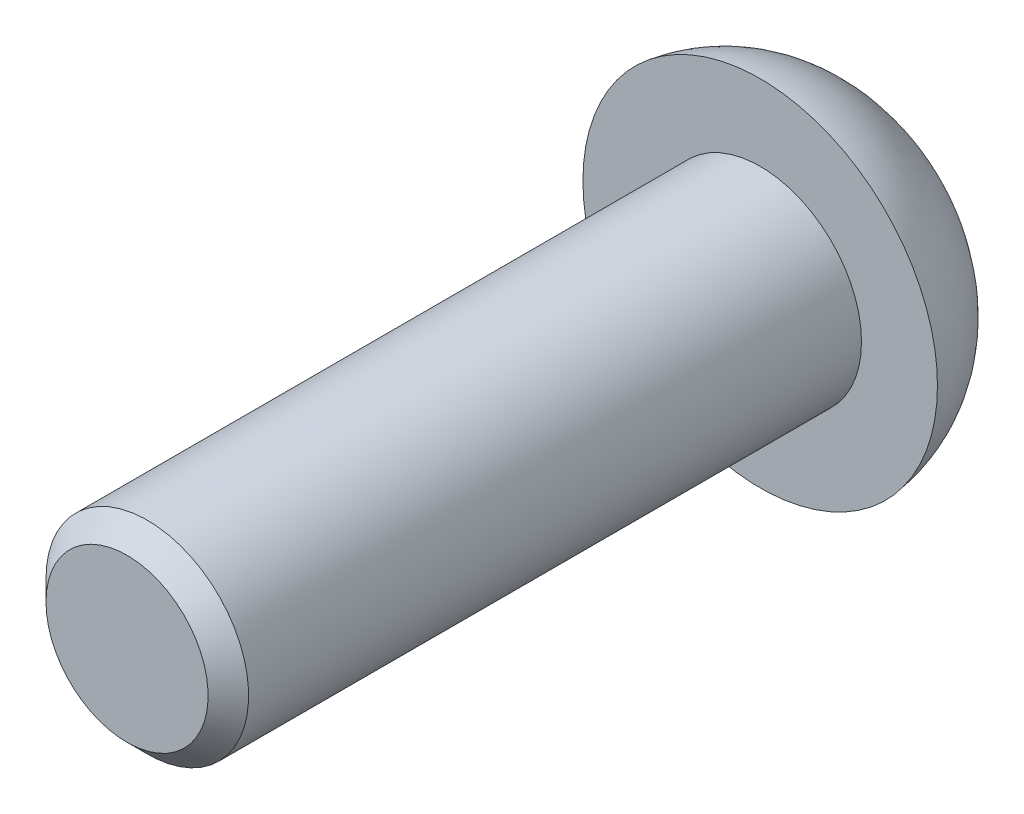
from build123d import *

# Parameters (mm, degrees)
SKETCH_1_R          = 7
EXTRUDE_1_DEPTH     = 4.4
SKETCH_2_R          = 4
EXTRUDE_2_DEPTH     = 25
CHAMFER_1_SIZE      = 0.8
CUT_EXTRUDE_1_DEPTH = 2.2


with BuildPart() as part:
    # 草图1 → 凸台-拉伸1 (new body)
    with BuildSketch(Plane.XY):
        Circle(SKETCH_1_R)
    extrude(amount=-EXTRUDE_1_DEPTH)

    # 草图2 → 凸台-拉伸2 (add)
    with BuildSketch(Plane(origin=(0, 0, 0), x_dir=(-1, 0, 0), z_dir=(0, 0, -1))):
        Circle(SKETCH_2_R)
    extrude(amount=-EXTRUDE_2_DEPTH)

    # 倒角1
    chamfer_1_edges = [part.edges().sort_by_distance(p)[0] for p in [
        (4, 0, 25),
    ]]
    chamfer(chamfer_1_edges, length=CHAMFER_1_SIZE)

    # 草图3 → 切除-拉伸1 (cut)
    with BuildSketch(Plane.XY.offset(-4.4)):
        Polygon((1.443375673, 2.5), (-1.443375673, 2.5), (-2.886751346, 0), (-1.443375673, -2.5), (1.443375673, -2.5), (2.886751346, 0), align=None)
    extrude(amount=CUT_EXTRUDE_1_DEPTH, mode=Mode.SUBTRACT)

    # 草图4 → 切除-旋转1 (revolve, cut)
    with BuildSketch(Plane(origin=(0, 0, 0), x_dir=(0, 1, 0), z_dir=(-1, 0, 0)), mode=Mode.PRIVATE) as cut_revolve_1_sk:
        Polygon((0, 0.756624327), (-2.5, 2.2), (0, 2.2), align=None)
    revolve(cut_revolve_1_sk.sketch.rotate(Axis((0, 0, 0), (0, 0, 1)), 270), axis=Axis((0, 0, 0), (0, 0, 1)), mode=Mode.SUBTRACT)

    # 草图5 → 切除-旋转2 (revolve, cut)
    with BuildSketch(Plane(origin=(0, 0, 0), x_dir=(1, 0, 0), z_dir=(0, 1, 0))):
        with BuildLine():
            Line((-7, 0), (-7, 4.4))
            Line((-7, 4.4), (-3.5, 4.4))
            ThreePointArc((-3.5, 4.4), (-5.867796506, 2.691429039), (-7, 0))
        make_face()
    revolve(axis=Axis((0, 0, 0), (0, 0, 1)), mode=Mode.SUBTRACT)


solid = part.part
